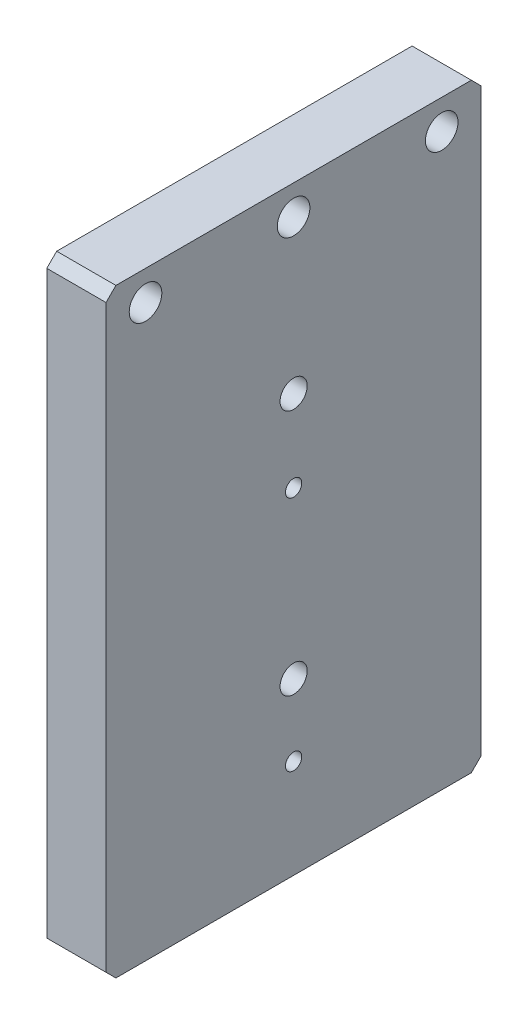
SolidWorks part; units mm, degrees
material "A6061"
ref_plane "前基準面" through (0, 0, 0) normal (0, 0, 1) x (1, 0, 0)
ref_plane "上基準面" through (0, 0, 0) normal (0, 1, 0) x (1, 0, 0)
ref_plane "右基準面" through (0, 0, 0) normal (1, 0, 0) x (0, 0, -1)
sketch "草图1" plane through (0, 0, 0) normal (1, 0, 0) x (0, 0, -1)
  line L1 (-38, 60.75) -> (38, 60.75)
  line L2 (-38, 60.75) -> (-38, -60.75)
  line L3 (-38, -60.75) -> (38, -60.75)
  line L4 (38, 60.75) -> (38, -60.75)
  line L5 (-38, 60.75) -> (38, -60.75) construction
  line L6 (-38, -60.75) -> (38, 60.75) construction
  point P0 (0, 0)
  dimension "D1" = 121.5
  dimension "D2" = 76
extrude "凸台-拉伸1" add sketch "草图1" along normal blind 12
sketch "草图7" plane through (0, 0, 0) normal (-1, 0, 0) x (0, 0, 1)
  line L1 (-38, 60.75) -> (38, 60.75) construction
  line L2 (0, 0) -> (0, 63.1593) construction
  point P0 (30, 54.75)
  point P2 (-30, 54.75)
  point P15 (0, 54.75)
  dimension "D1" = 60
  dimension "D3" = 6
hole_wizard "M6 六角圆柱头螺钉的柱形沉头孔1" positions "草图7" profile "草图8" counterbore size "M6" standard "GB" end condition through all
sketch "草图8" plane through (0, 54.75, 30) normal (0, 1, 0) x (0, 0, 1)
  line L0 (0, 0) -> (0, 12)
  line L1 (0, 12) -> (3.3, 12)
  line L3 (3.3, 12) -> (3.3, 6.8)
  line L4 (3.3, 6.8) -> (5.5, 6.8)
  line L5 (5.5, 6.8) -> (5.5, 0)
  line L7 (5.5, 0) -> (0, 0)
  line L11 (0, -6.35) -> (0, 107.95) construction
  dimension "通孔孔直径" = 6.6
  dimension "通孔孔深度" = 12
  dimension "柱形沉头孔直径" = 11
  dimension "柱形沉头孔深度" = 6.8
sketch "草图9" plane through (0, 0, 0) normal (-1, 0, 0) x (0, 0, 1)
  line L3 (38, -60.75) -> (-38, -60.75) construction
  line L5 (0, 0) -> (0, -67.3431) construction
  point P6 (0, 7.25)
  point P9 (0, -40.75)
  dimension "D3" = 48
  dimension "D4" = 20
hole_wizard "M4 螺纹孔1" positions "草图9" profile "草图10" tap size "M4" standard "GB" end condition through all
sketch "草图10" plane through (0, 7.25, 0) normal (0, 1, 0) x (0, 0, 1)
  line L0 (0, 0) -> (0, 12)
  line L1 (0, 12) -> (1.65, 12)
  line L2 (1.65, 12) -> (1.65, 0)
  line L5 (1.65, 0) -> (0, 0)
  line L11 (0, -6.35) -> (0, 107.95) construction
  dimension "通孔螺纹孔钻头直径" = 3.3
  dimension "通孔螺纹孔钻头深度" = 12
cosmetic thread "孔螺纹线3" parameters "D2"=4
cosmetic thread "孔螺纹线4" parameters "D2"=4
hole_wizard "Ø5.0mm 暗销孔1" positions "草图3" profile "草图4" hole size "Ø5.0" standard "GB"
sketch "草图3" plane through (0, 0, 0) normal (-1, 0, 0) x (0, 0, 1)
  line L0 (0, -40.75) -> (43.0426, -40.75) construction
  line L3 (0, 7.25) -> (41.9098, 7.25) construction
  line L4 (0, 7.25) -> (0, -67.0394) construction
  circle A0 centre (0, 7.25) radius 1.65 construction
  point P24 (24, 7.25)
  point P26 (24, -40.75)
  point P52 (-24, -40.75)
  point P53 (-24, 7.25)
  dimension "D1" = 24
sketch "草图4" plane through (0, 7.25, 24) normal (0, 1, 0) x (0, 0, 1)
  line L0 (0, 0) -> (0, 7.5022)
  line L1 (0, 7.5022) -> (2.5, 6)
  line L2 (2.5, 6) -> (2.5, 0)
  line L5 (2.5, 0) -> (0, 0)
  line L10 (0, 7.5022) -> (-2.5, 6) construction
  line L11 (0, -6.35) -> (0, 107.95) construction
  dimension "孔直径" = 5
  dimension "孔深度" = 6
  dimension "导头角度" = 118
hole_wizard "M5 六角圆柱头螺钉的柱形沉头孔1" positions "草图11" profile "草图12" counterbore size "M5" standard "GB"
sketch "草图11" plane through (0, 0, 0) normal (-1, 0, 0) x (0, 0, 1)
  point P0 (0, 23.75)
  point P2 (0, -26.25)
sketch "草图12" plane through (0, 23.75, 0) normal (0, 1, 0) x (0, 0, 1)
  line L0 (0, 0) -> (0, 14.0524)
  line L1 (0, 14.0524) -> (2.75, 12.4)
  line L2 (2.75, 12.4) -> (2.75, 5.7)
  line L3 (2.75, 5.7) -> (5, 5.7)
  line L4 (5, 5.7) -> (5, 0)
  line L5 (5, 0) -> (0, 0)
  line L10 (0, 14.0524) -> (-2.75, 12.4) construction
  line L11 (0, -6.35) -> (0, 107.95) construction
  dimension "孔直径" = 5.5
  dimension "孔深度" = 12.4
  dimension "柱形沉头孔直径" = 10
  dimension "柱形沉头孔深度" = 5.7
  dimension "导头角度" = 118
chamfer "倒角1" distance 2 angle 45 4 edges at (6, -60.75, 38) (6, 60.75, 38) (6, -60.75, -38) (6, 60.75, -38)
